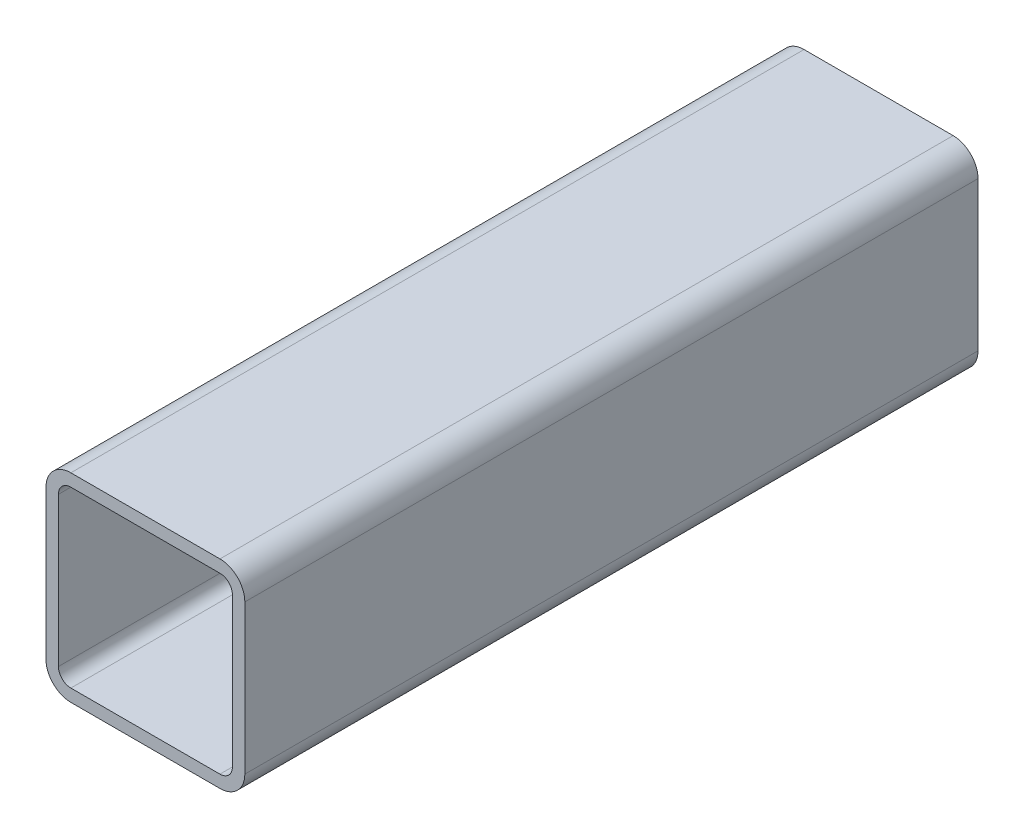
SolidWorks part; units mm, degrees
ref_plane "Front Plane" through (0, 0, 0) normal (0, 0, 1) x (1, 0, 0)
ref_plane "Top Plane" through (0, 0, 0) normal (0, 1, 0) x (1, 0, 0)
ref_plane "Right Plane" through (0, 0, 0) normal (1, 0, 0) x (0, 0, -1)
sketch "Sketch 1" plane through (0, 0, 0) normal (0, 0, 1) x (1, 0, 0)
  line L0 (0, 96.8978) -> (0, -107.4818) construction
  line L1 (-129.1971, 0) -> (137.9562, 0) construction
  line L2 (0, 32) -> (-24, 32)
  line L3 (-32, 24) -> (-32, 0)
  line L4 (0, 28) -> (-24, 28)
  line L5 (-28, 24) -> (-28, 0)
  line L6 (-28, -24) -> (-28, 0)
  line L7 (24, -28) -> (-24, -28)
  line L8 (-32, -24) -> (-32, 0)
  line L9 (24, -32) -> (-24, -32)
  line L10 (32, -24) -> (32, 0)
  line L11 (28, -24) -> (28, 0)
  line L12 (28, 24) -> (28, 0)
  line L13 (0, 28) -> (24, 28)
  line L14 (32, 24) -> (32, 0)
  line L15 (0, 32) -> (24, 32)
  arc A0 (-24, 32) -> (-32, 24) centre (-24, 24) ccw
  arc A1 (-24, 28) -> (-28, 24) centre (-24, 24) ccw
  arc A2 (-24, -28) -> (-28, -24) centre (-24, -24) cw
  arc A3 (-24, -32) -> (-32, -24) centre (-24, -24) cw
  arc A4 (24, -32) -> (32, -24) centre (24, -24) ccw
  arc A5 (24, -28) -> (28, -24) centre (24, -24) ccw
  arc A6 (24, 28) -> (28, 24) centre (24, 24) cw
  arc A7 (24, 32) -> (32, 24) centre (24, 24) cw
  point P34 (0, -32)
  point P35 (0, -28)
  dimension "D3" = 8
  dimension "D1" = 64
  dimension "D2" = 64
  dimension "D4" = 4
extrude "Boss-Extrude 1" add sketch "Sketch 1" along normal mid plane 236
